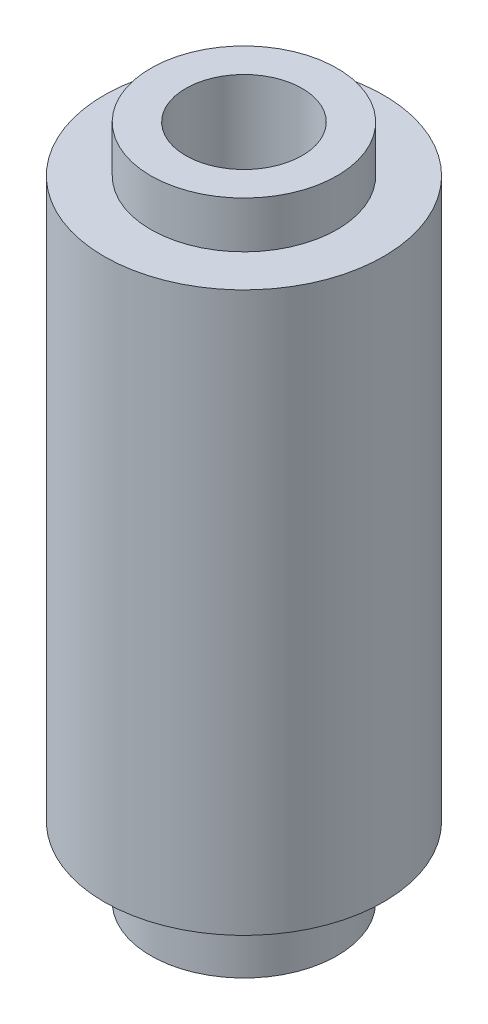
from build123d import *

# Parameters (mm, degrees)
SKETCH_2_R           = 3
BOSS_EXTRUDE_1_DEPTH = 12
SKETCH_3_R           = 2
BOSS_EXTRUDE_2_DEPTH = 1
BOSS_EXTRUDE_START   = 1.5
SKETCH_4_R           = 2
BOSS_EXTRUDE_3_DEPTH = 1.5
SKETCH_5_R           = 1.25
CUT_EXTRUDE_1_DEPTH  = 6
SKETCH_6_R           = 1.5
CUT_EXTRUDE_2_DEPTH  = 2.5
CUT_EXTRUDE_3_DEPTH  = 6
CUT_EXTRUDE_START    = -0.43115
SKETCH_11_R          = 0.5
CUT_EXTRUDE_8_DEPTH  = 1.93115


with BuildPart() as part:
    # Sketch 2 → Boss-Extrude 1 (new body)
    with BuildSketch(Plane(origin=(0, 0, 0), x_dir=(1, 0, 0), z_dir=(0, 1, 0))):
        with Locations(Location((0, 0, 0), (0, 0, 270))):
            Circle(SKETCH_2_R)
    extrude(amount=BOSS_EXTRUDE_1_DEPTH)

    # Sketch 3 → Boss-Extrude 2 (add)
    with BuildSketch(Plane(origin=(0, 12, 0), x_dir=(1, 0, 0), z_dir=(0, 1, 0))):
        with Locations(Location((0, 0, 0), (0, 0, 270))):
            Circle(SKETCH_3_R)
    extrude(amount=BOSS_EXTRUDE_2_DEPTH)

    # Sketch 4 → Boss-Extrude 3 (add)
    with BuildSketch(Plane(origin=(0, 0, 0), x_dir=(-1, 0, 0), z_dir=(0, -1, 0)).offset(BOSS_EXTRUDE_START)):
        with Locations(Location((0, 0, 0), (0, 0, 270))):
            Circle(SKETCH_4_R)
    extrude(amount=-BOSS_EXTRUDE_3_DEPTH)

    # Sketch 5 → Cut-Extrude 1 (cut)
    with BuildSketch(Plane(origin=(0, 13, 0), x_dir=(1, 0, 0), z_dir=(0, 1, 0))):
        with Locations(Location((0, 0, 0), (0, 0, 270))):
            Circle(SKETCH_5_R)
    extrude(amount=-CUT_EXTRUDE_1_DEPTH, mode=Mode.SUBTRACT)

    # Sketch 6 → Cut-Extrude 2 (cut)
    with BuildSketch(Plane(origin=(0, 7, 0), x_dir=(1, 0, 0), z_dir=(0, 1, 0))):
        with Locations(Location((0, 0, 0), (0, 0, 270))):
            Circle(SKETCH_6_R)
    extrude(amount=-CUT_EXTRUDE_2_DEPTH, mode=Mode.SUBTRACT)

    # Sketch 7 → Cut-Extrude 3 (cut)
    with BuildSketch(Plane(origin=(0, -1.5, 0), x_dir=(-1, 0, 0), z_dir=(0, -1, 0))):
        Polygon((-0.97407891, 1.14068851), (-1.385866178, -0.57391196), (0.117566508, -1.495385608), (1.458526276, -0.350287172), (0.783852304, 1.27889623), align=None)
    extrude(amount=-CUT_EXTRUDE_3_DEPTH, mode=Mode.SUBTRACT)

    # Sketch 11 → Cut-Extrude 8 (cut)
    with BuildSketch(Plane(origin=(-0.783852304, 0, -1.27889623), x_dir=(-0.8525974863360001, 0, 0.5225682025281811), z_dir=(-0.5225682025281811, 0, -0.8525974863360001)).offset(CUT_EXTRUDE_START)):
        with Locations(Location((-0.093426493, 1.5893341, 0), (0, 0, 180))):
            Circle(SKETCH_11_R)
    extrude(amount=CUT_EXTRUDE_8_DEPTH, mode=Mode.SUBTRACT)


solid = part.part
